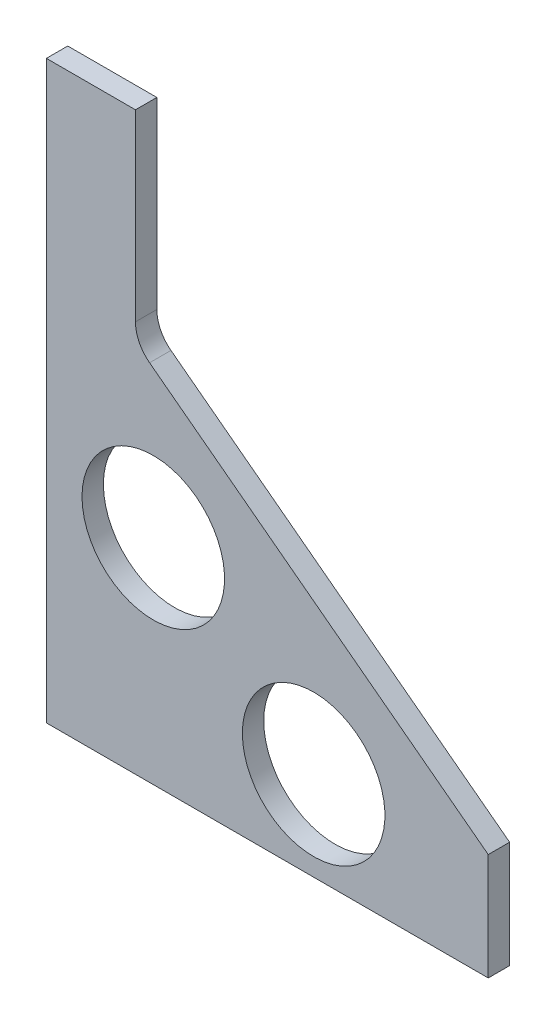
from build123d import *

# Parameters (mm, degrees)
SKETCH_1_W             = 248
SKETCH_1_H             = 60
EXTRUDE_1_DEPTH        = 6
EXTRUDE_2_DEPTH        = 12
FILLET_1_R             = 20
SKETCH_3_R             = 40
CUT_EXTRUDE_1_DEPTH    = 319.384987083
HOLE_WIZARD_M5_1_D     = 4.2
HOLE_WIZARD_M5_1_DEPTH = 12.4
HOLE_WIZARD_M5_1_TIP   = 1.2618073
HOLE_WIZARD_M5_2_D     = 4.2
HOLE_WIZARD_M5_2_DEPTH = 12.4
HOLE_WIZARD_M5_2_TIP   = 1.2618073


with BuildPart() as part:
    # 草图1 → 凸台-拉伸1 (new, symmetric)
    with BuildSketch(Plane.XY):
        Rectangle(SKETCH_1_W, SKETCH_1_H)
    extrude(amount=EXTRUDE_1_DEPTH, both=True)

    # 草图2 → 凸台-拉伸2 (add)
    with BuildSketch(Plane(origin=(0, 0, -6), x_dir=(-1, 0, 0), z_dir=(0, 0, -1))):
        Polygon((-124, 30), (74, 180), (74, 293), (124, 293), (124, 30), align=None)
    extrude(amount=-EXTRUDE_2_DEPTH)

    # 圆角1
    fillet_1_edges = [part.edges().sort_by_distance(p)[0] for p in [
        (-74, 180, 0),
    ]]
    fillet(fillet_1_edges, radius=FILLET_1_R)

    # 草图3 → 切除-拉伸1 (cut, through all)
    with BuildSketch(Plane(origin=(0, 0, -6), x_dir=(-1, 0, 0), z_dir=(0, 0, -1))):
        with Locations((-26, 20)):
            Circle(SKETCH_3_R)
        with Locations((64, 90)):
            Circle(SKETCH_3_R)
    extrude(amount=-CUT_EXTRUDE_1_DEPTH, mode=Mode.SUBTRACT)

    # M5 螺纹孔1
    with Locations(Plane(origin=(0, -30, 0), x_dir=(-1, 0, 0), z_dir=(0, -1, 0))):
        with Locations((-90, 0), (0, 0), (90, 0)):
            Hole(HOLE_WIZARD_M5_1_D / 2, depth=HOLE_WIZARD_M5_1_DEPTH)
            with Locations((0, 0, -(HOLE_WIZARD_M5_1_DEPTH + HOLE_WIZARD_M5_1_TIP / 2))):  # 118° drill point
                Cone(0, HOLE_WIZARD_M5_1_D / 2, HOLE_WIZARD_M5_1_TIP, mode=Mode.SUBTRACT)

    # M5 螺纹孔2
    with Locations(Plane.ZY.offset(124)):
        with Locations((0, 238), (0, 128), (0, 18)):
            Hole(HOLE_WIZARD_M5_2_D / 2, depth=HOLE_WIZARD_M5_2_DEPTH)
            with Locations((0, 0, -(HOLE_WIZARD_M5_2_DEPTH + HOLE_WIZARD_M5_2_TIP / 2))):  # 118° drill point
                Cone(0, HOLE_WIZARD_M5_2_D / 2, HOLE_WIZARD_M5_2_TIP, mode=Mode.SUBTRACT)


solid = part.part
